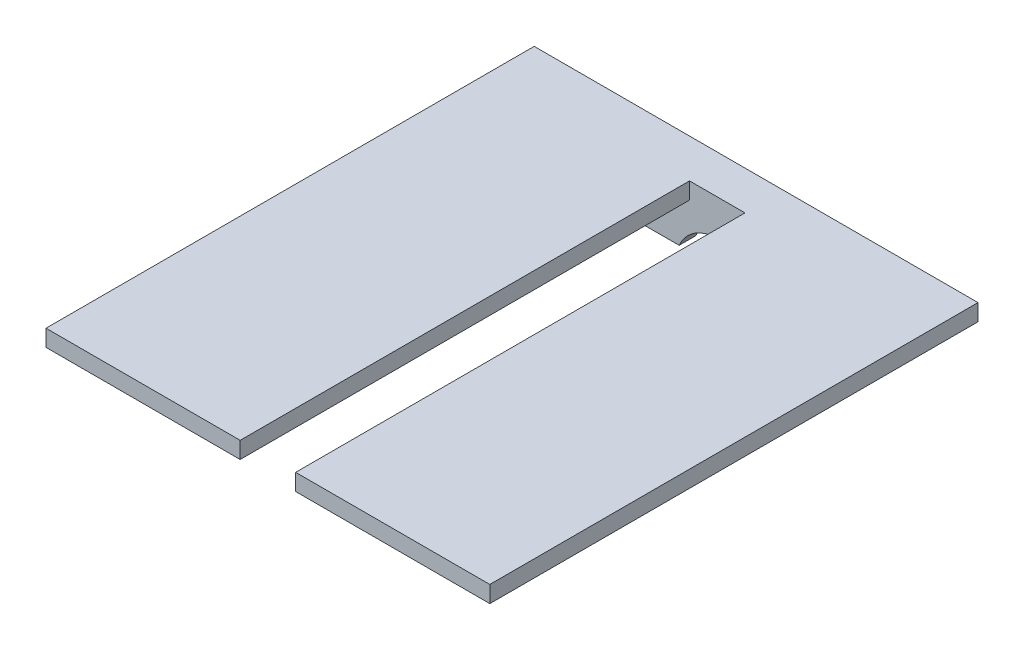
from build123d import *

# Parameters (mm, degrees)
SKETCH2_R           = 1.5
BOSS_EXTRUDE1_DEPTH = 3
BOSS_EXTRUDE2_DEPTH = 3


with BuildPart() as part:
    # Sketch2 → Boss-Extrude1 (new body)
    with BuildSketch(Plane.XY):
        with BuildLine():
            Line((-20, 3), (-6.873863542, 3))
            ThreePointArc((-6.873863542, 3), (0, 7.5), (6.873863542, 3))
            Line((6.873863542, 3), (20, 3))
            Line((20, 3), (20, 11))
            Line((20, 11), (-20, 11))
            Line((-20, 11), (-20, 3))
        make_face()
        with Locations((-17, 7)):
            Circle(SKETCH2_R, mode=Mode.SUBTRACT)
        with Locations((17, 7)):
            Circle(SKETCH2_R, mode=Mode.SUBTRACT)
    extrude(amount=BOSS_EXTRUDE1_DEPTH)

    # Sketch3 → Boss-Extrude2 (add)
    with BuildSketch(Plane(origin=(0, 11, 0), x_dir=(1, 0, 0), z_dir=(0, 1, 0))):
        Polygon((-5, -84), (-40, -84), (-40, 0), (-40, 4), (40, 4), (40, 0), (40, -84), (5, -84), (5, -3), (-5, -3), align=None)
    extrude(amount=BOSS_EXTRUDE2_DEPTH)


solid = part.part
